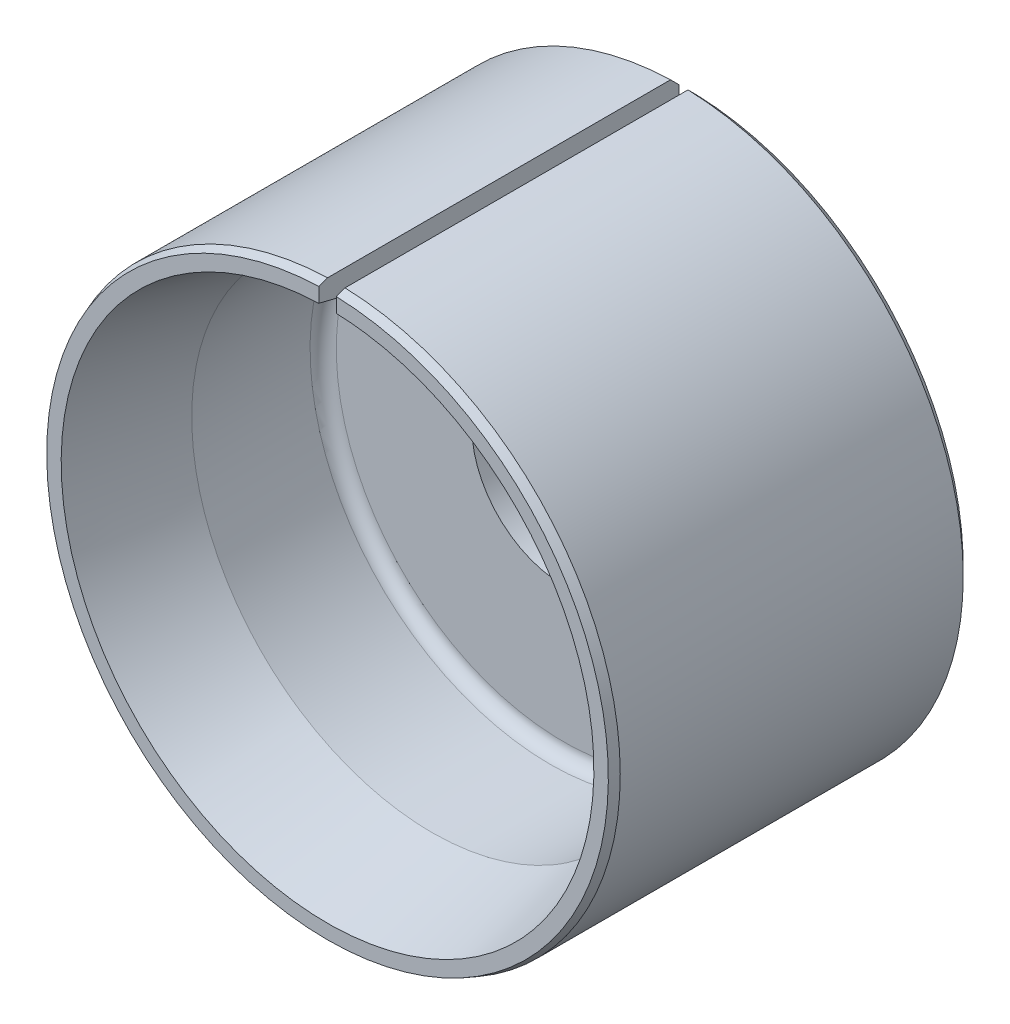
from build123d import *

# Parameters (mm, degrees)
SKETCH_1_R          = 32.5
EXTRUDE_1_DEPTH     = 41.25
SKETCH_2_R          = 27.5
CUT_EXTRUDE_1_DEPTH = 27
HOLE_WIZARD_M24_1_D = 21
SKETCH_4_W          = 2
SKETCH_4_H          = 41.62847608
CUT_EXTRUDE_2_DEPTH = 62.758096635
CHAMFER_1_SIZE      = 1
CHAMFER_2_SIZE      = 1
CHAMFER_2_SIZE2     = 0.363970234
FILLET_1_R          = 1.5


with BuildPart() as part:
    # 草图1 → 凸台-拉伸1 (new body)
    with BuildSketch(Plane.XY):
        Circle(SKETCH_1_R)
    extrude(amount=EXTRUDE_1_DEPTH)

    # 草图2 → 切除-拉伸1 (cut)
    with BuildSketch(Plane.XY.offset(41.25)):
        Circle(SKETCH_2_R)
    extrude(amount=-CUT_EXTRUDE_1_DEPTH, mode=Mode.SUBTRACT)

    # M24 螺纹孔1 (through all)
    with Locations(Plane(origin=(0, 0, 0), x_dir=(-1, 0, 0), z_dir=(0, 0, -1))):
        with Locations((0, 0)):
            Hole(HOLE_WIZARD_M24_1_D / 2)

    # 草图4 → 切除-拉伸2 (cut, through all)
    with BuildSketch(Plane(origin=(0, 0, 0), x_dir=(-1, 0, 0), z_dir=(0, 0, -1))):
        with Locations((0, 16.25)):
            Rectangle(SKETCH_4_W, SKETCH_4_H)
    extrude(amount=-CUT_EXTRUDE_2_DEPTH, mode=Mode.SUBTRACT)

    # 草图5 → 切除-旋转1 (revolve, cut)
    with BuildSketch(Plane(origin=(0, 0, 0), x_dir=(0, 0, -1), z_dir=(1, 0, 0))):
        Polygon((-44.25, 27.481812167), (-29.25, 27.481812167), (-44.25, 31.22173221), align=None)
    revolve(axis=Axis((0, -0.007694129, 41.25), (0, 0.00018652434146350927, -0.9999999826043349)), mode=Mode.SUBTRACT)

    # 倒角1
    chamfer_1_edges = [part.edges().sort_by_distance(p)[0] for p in [
        (-22.624654693, -23.331845191, 0),
    ]]
    chamfer(chamfer_1_edges, length=CHAMFER_1_SIZE)

    # 倒角2
    chamfer_2_edges = [part.edges().sort_by_distance(p)[0] for p in [
        (-22.624654693, -23.331845191, 41.25),
    ]]
    chamfer_2_side = [part.faces().sort_by_distance(p)[0] for p in [
        (-22.624654693, -23.331845191, 21.125),
    ]]
    chamfer(chamfer_2_edges, length=CHAMFER_2_SIZE, length2=CHAMFER_2_SIZE2, reference=chamfer_2_side[0])

    # 圆角1
    fillet_1_edges = [part.edges().sort_by_distance(p)[0] for p in [
        (-19.088609169, -19.795832895, 14.25),
    ]]
    fillet(fillet_1_edges, radius=FILLET_1_R)


solid = part.part
